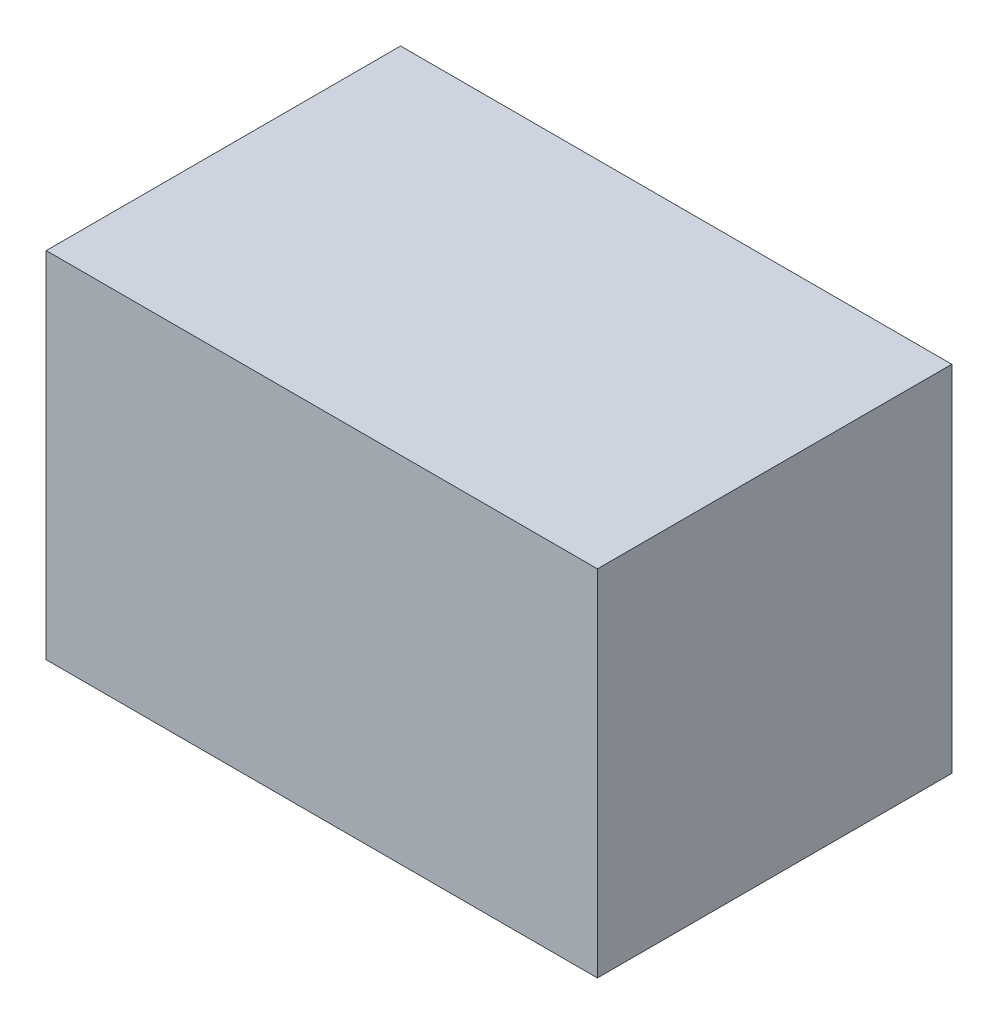
from build123d import *

# Parameters (mm, degrees)
SKETCH_1_W      = 140
SKETCH_1_H      = 90
EXTRUDE_1_DEPTH = 45


with BuildPart() as part:
    # 草图1 → 凸台-拉伸1 (new, symmetric)
    with BuildSketch(Plane.XY):
        Rectangle(SKETCH_1_W, SKETCH_1_H)
    extrude(amount=EXTRUDE_1_DEPTH, both=True)


solid = part.part
